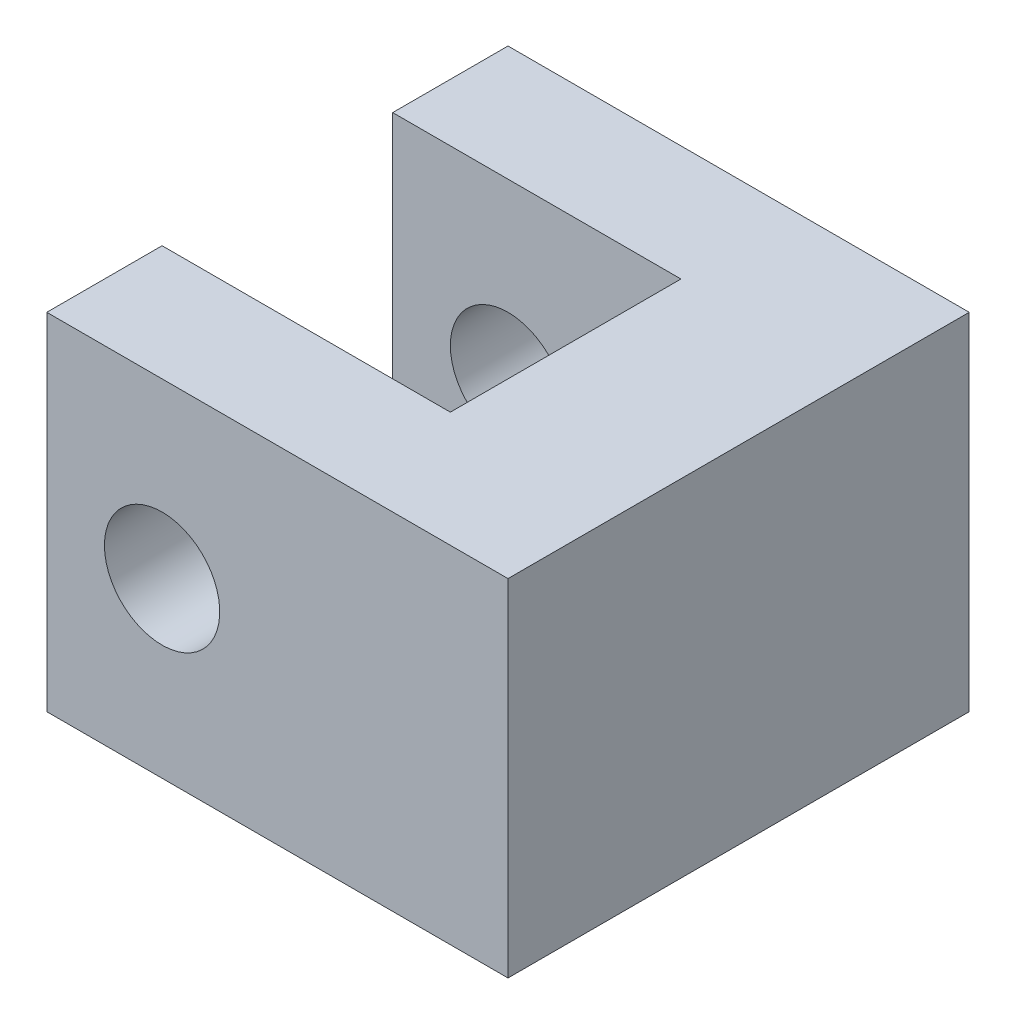
SolidWorks part; units mm, degrees
ref_plane "Front Plane" through (0, 0, 0) normal (0, 0, 1) x (1, 0, 0)
ref_plane "Top Plane" through (0, 0, 0) normal (0, 1, 0) x (1, 0, 0)
ref_plane "Right Plane" through (0, 0, 0) normal (1, 0, 0) x (0, 0, -1)
sketch "Sketch1" plane through (0, 0, 0) normal (0, 1, 0) x (1, 0, 0)
  line L0 (-20, 10) -> (-20, 20)
  line L1 (-20, -20) -> (20, -20)
  line L2 (-20, -20) -> (-20, -10)
  line L3 (-20, 20) -> (20, 20)
  line L4 (20, -20) -> (20, 20)
  line L5 (-20, -20) -> (20, 20) construction
  line L6 (-20, 20) -> (20, -20) construction
  line L7 (-20, 10) -> (5, 10)
  line L9 (-20, -10) -> (5, -10)
  line L10 (5, 10) -> (5, -10)
  point P0 (0, 0)
  dimension "D1" = 40
  dimension "D2" = 40
  dimension "D3" = 20
  dimension "D4" = 10
  dimension "D5" = 25
extrude "Boss-Extrude1" add sketch "Sketch1" along normal blind 30
sketch "Sketch2" plane through (0, 0, -20) normal (0, 0, -1) x (-1, 0, 0)
  line L0 (-20, 30) -> (20, 30) construction
  line L1 (20, 30) -> (20, 0) construction
  circle A0 centre (10, 15) radius 5
  dimension "D1" = 10
  dimension "D2" = 15
  dimension "D3" = 10
extrude "Cut-Extrude1" cut sketch "Sketch2" against normal through all
